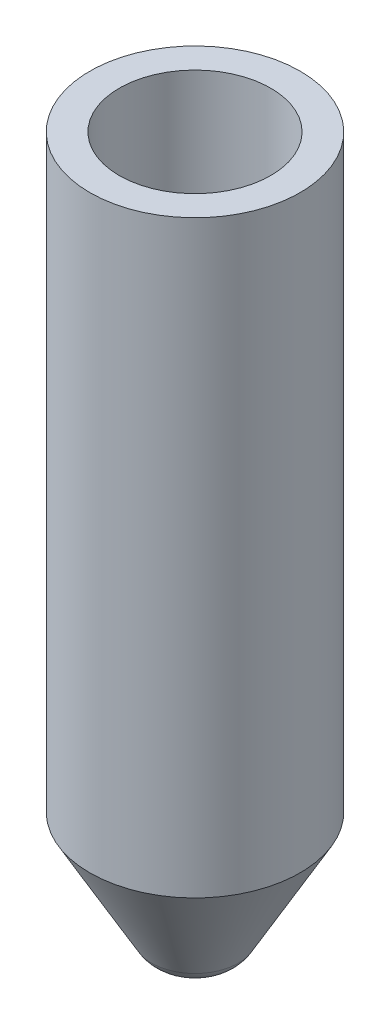
from build123d import *

# Parameters (mm, degrees)
FILLET1_R = 80
SHELL1_T  = -70


with BuildPart() as part:
    # Sketch2 → Revolve1 (revolve)
    with BuildSketch(Plane.XY, mode=Mode.PRIVATE) as revolve1_sk:
        Polygon((0, 1700), (250, 1700), (250, 300), (80, 0), (0, 0), align=None)
    revolve(revolve1_sk.sketch.rotate(Axis((0, 0, 0), (0, 1, 0)), 270), axis=Axis((0, 0, 0), (0, 1, 0)))

    # Fillet1
    fillet1_edges = [part.edges().sort_by_distance(p)[0] for p in [
        (0, 0, -80),
    ]]
    fillet(fillet1_edges, radius=FILLET1_R)

    # Shell1
    shell1_openings = [part.faces().sort_by_distance(p)[0] for p in [
        (0, 1700, 0),
    ]]
    offset(amount=SHELL1_T, openings=shell1_openings, kind=Kind.INTERSECTION)


solid = part.part
